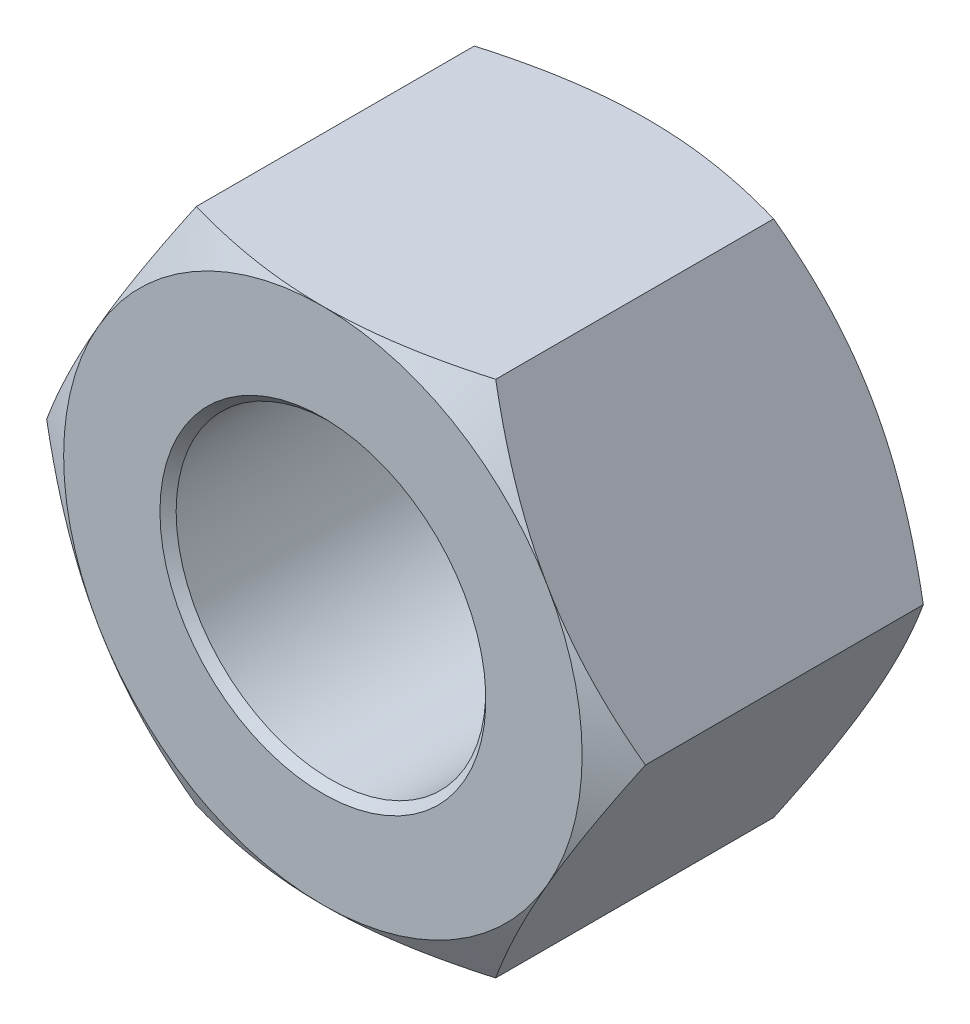
SolidWorks part; units mm, degrees
ref_plane "基准面1" through (0, 0, 0) normal (0, 0, 1) x (1, 0, 0)
ref_plane "基准面2" through (0, 0, 0) normal (0, 1, 0) x (1, 0, 0)
ref_plane "基准面3" through (0, 0, 0) normal (1, 0, 0) x (0, 0, -1)
sketch "尺寸草图" plane through (0, 0, 0) normal (0, 0, 1) x (1, 0, 0)
  line L0 (0, 0) -> (34, 0) construction
  point P1 (31.4, 0)
  point P3 (22, 0)
  point P4 (2.5, 0)
  point P5 (37.3, 0)
  point P6 (20.2, 0)
  point P8 (34, 0)
  dimension "D" = 22
  dimension "e(最小)" = 37.3
  dimension "m(最大)" = 20.2
  dimension "s(公称)" = 34
  dimension "dw(最小)" = 31.4
  dimension "P" = 2.5
sketch "草图1" plane through (0, 0, 0) normal (0, 0, 1) x (1, 0, 0)
  line L0 (-26.8088, 0) -> (37.1748, 0) construction
  line L1 (0, 25.0215) -> (0, -25.0215) construction
  line L3 (9.325, 16.1514) -> (-9.325, 16.1514)
  line L4 (-9.325, 16.1514) -> (-18.65, 0)
  line L5 (-18.65, 0) -> (-9.325, -16.1514)
  line L6 (-9.325, -16.1514) -> (9.325, -16.1514)
  line L7 (9.325, -16.1514) -> (18.65, 0)
  line L8 (18.65, 0) -> (9.325, 16.1514)
  circle A0 centre (0, 0) radius 16.1514 construction
  circle A1 centre (0, 0) radius 9.6469
  dimension "D" = 19.2937
  dimension "e" = 37.3
extrude "基体-拉伸" add sketch "草图1" along normal blind 20.2
cosmetic thread "装饰螺纹线1" parameters "D2"=22
sketch "草图2" plane through (0, 0, 0) normal (0, 0, -1) x (-1, 0, 0)
  line L0 (-9.325, 16.1514) -> (9.325, 16.1514) construction
  circle A0 centre (0, 0) radius 16.1514
  circle A1 centre (0, 0) radius 9.6469 construction
extrude "切除-拉伸1" cut sketch "草图2" against normal through all draft 60 flip side to cut
sketch "草图3" plane through (0, 0, 20.2) normal (0, 0, 1) x (1, 0, 0)
  line L0 (18.65, 0) -> (9.325, 16.1514) construction
  circle A0 centre (0, 0) radius 16.1514
extrude "切除-拉伸2" cut sketch "草图3" against normal through all draft 60 flip side to cut
chamfer "倒角1" distance 0.505 angle 45 2 edges at (9.6469, 0, 0) (9.6469, 0, 20.2)
